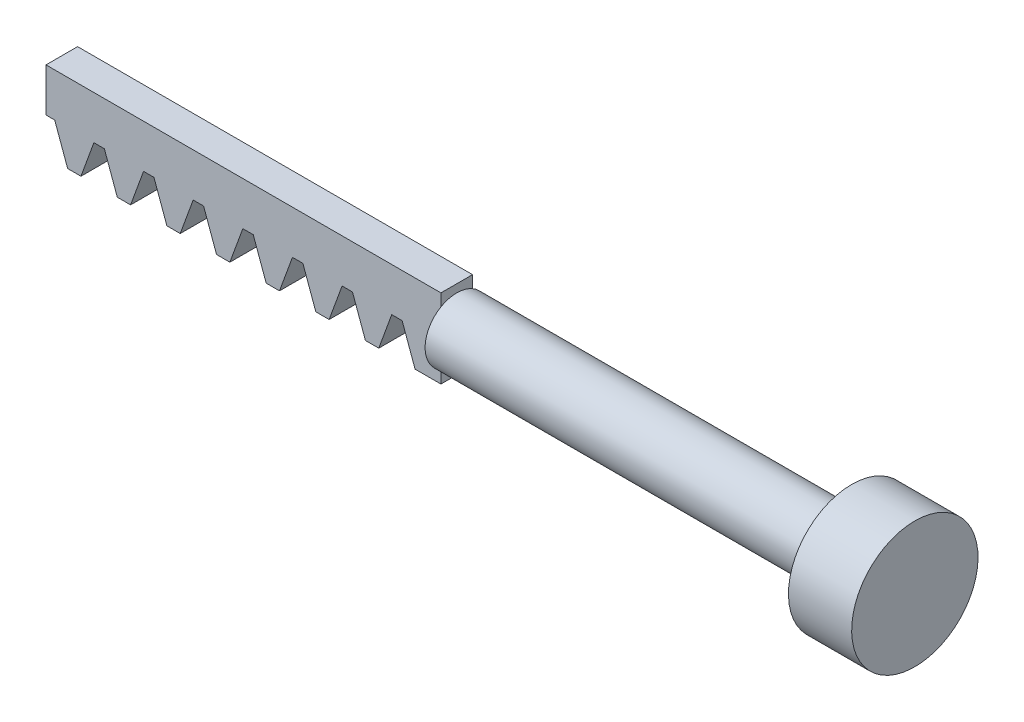
SolidWorks part; units mm, degrees
ref_plane "Front Plane" through (0, 0, 0) normal (0, 0, 1) x (1, 0, 0)
ref_plane "Top Plane" through (0, 0, 0) normal (0, 1, 0) x (1, 0, 0)
ref_plane "Right Plane" through (0, 0, 0) normal (1, 0, 0) x (0, 0, -1)
ref_plane "Plane1" through (0, 0, 2) normal (0, 0, 1) x (1, 0, 0)
sketch "Sketch1" plane through (0, 0, 2) normal (0, 0, 1) x (1, 0, 0)
  line L0 (-50, 10) -> (-50, 0)
  line L1 (-50, 0) -> (0, 0)
  line L2 (0, 0) -> (0, 10)
  line L3 (0, 10) -> (-50, 10)
extrude "Boss-Extrude1" add sketch "Sketch1" against normal blind 4
sketch "Sketch2" plane through (0, 0, -2) normal (0, 0, -1) x (-1, 0, 0)
  line L0 (40.9761, 0) -> (45.5739, 0)
  line L1 (45.5739, 0) -> (43.9361, 4.5)
  line L2 (43.9361, 4.5) -> (42.6139, 4.5)
  line L3 (42.6139, 4.5) -> (40.9761, 0)
extrude "Cut-Extrude1" cut sketch "Sketch2" against normal through all
sketch "Sketch3" plane through (0, 0, -2) normal (0, 0, -1) x (-1, 0, 0)
  line L0 (34.6921, 0) -> (39.2899, 0)
  line L1 (39.2899, 0) -> (37.6521, 4.5)
  line L2 (37.6521, 4.5) -> (36.3299, 4.5)
  line L3 (36.3299, 4.5) -> (34.6921, 0)
extrude "Cut-Extrude2" cut sketch "Sketch3" against normal through all
sketch "Sketch4" plane through (0, 0, -2) normal (0, 0, -1) x (-1, 0, 0)
  line L0 (28.4081, 0) -> (33.0059, 0)
  line L1 (33.0059, 0) -> (31.3681, 4.5)
  line L2 (31.3681, 4.5) -> (30.0459, 4.5)
  line L3 (30.0459, 4.5) -> (28.4081, 0)
extrude "Cut-Extrude3" cut sketch "Sketch4" against normal through all
sketch "Sketch5" plane through (0, 0, -2) normal (0, 0, -1) x (-1, 0, 0)
  line L0 (22.1241, 0) -> (26.7219, 0)
  line L1 (26.7219, 0) -> (25.0841, 4.5)
  line L2 (25.0841, 4.5) -> (23.7619, 4.5)
  line L3 (23.7619, 4.5) -> (22.1241, 0)
extrude "Cut-Extrude4" cut sketch "Sketch5" against normal through all
sketch "Sketch6" plane through (0, 0, -2) normal (0, 0, -1) x (-1, 0, 0)
  line L0 (15.8401, 0) -> (20.4379, 0)
  line L1 (20.4379, 0) -> (18.8001, 4.5)
  line L2 (18.8001, 4.5) -> (17.4779, 4.5)
  line L3 (17.4779, 4.5) -> (15.8401, 0)
extrude "Cut-Extrude5" cut sketch "Sketch6" against normal through all
sketch "Sketch7" plane through (0, 0, -2) normal (0, 0, -1) x (-1, 0, 0)
  line L0 (9.5561, 0) -> (14.1539, 0)
  line L1 (14.1539, 0) -> (12.5161, 4.5)
  line L2 (12.5161, 4.5) -> (11.1939, 4.5)
  line L3 (11.1939, 4.5) -> (9.5561, 0)
extrude "Cut-Extrude6" cut sketch "Sketch7" against normal through all
sketch "Sketch8" plane through (0, 0, -2) normal (0, 0, -1) x (-1, 0, 0)
  line L0 (3.2721, 0) -> (7.8699, 0)
  line L1 (7.8699, 0) -> (6.2321, 4.5)
  line L2 (6.2321, 4.5) -> (4.9099, 4.5)
  line L3 (4.9099, 4.5) -> (3.2721, 0)
extrude "Cut-Extrude7" cut sketch "Sketch8" against normal through all
sketch "Sketch9" plane through (0, 0, -2) normal (0, 0, -1) x (-1, 0, 0)
  line L0 (48.8979, 4.5) -> (47.2601, 0)
  line L1 (47.2601, 0) -> (50, 0)
  line L2 (50, 0) -> (50, 4.5)
  line L3 (50, 4.5) -> (48.8979, 4.5)
extrude "Cut-Extrude8" cut sketch "Sketch9" against normal through all
sketch "Sketch10" plane through (0, 0, 0) normal (0, 0, 1) x (1, 0, 0)
  line L0 (0, 9) -> (0, 5)
  line L1 (0, 5) -> (58, 5)
  line L2 (58, 5) -> (58, 13)
  line L3 (58, 13) -> (50, 13)
  line L4 (50, 13) -> (50, 9)
  line L5 (50, 9) -> (0, 9)
  line L6 (0, 5) -> (58, 5) construction
revolve "Revolve1" add sketch "Sketch10" angle 360 about L6
sketch "Sketch11" plane through (0, 0, 2) normal (0, 0, 1) x (1, 0, 0)
  line L0 (-56.5531, 2) -> (12.0925, 2)
  line L4 (-47.2601, 0) -> (-45.5739, 0) construction
  dimension "D1" = 2
